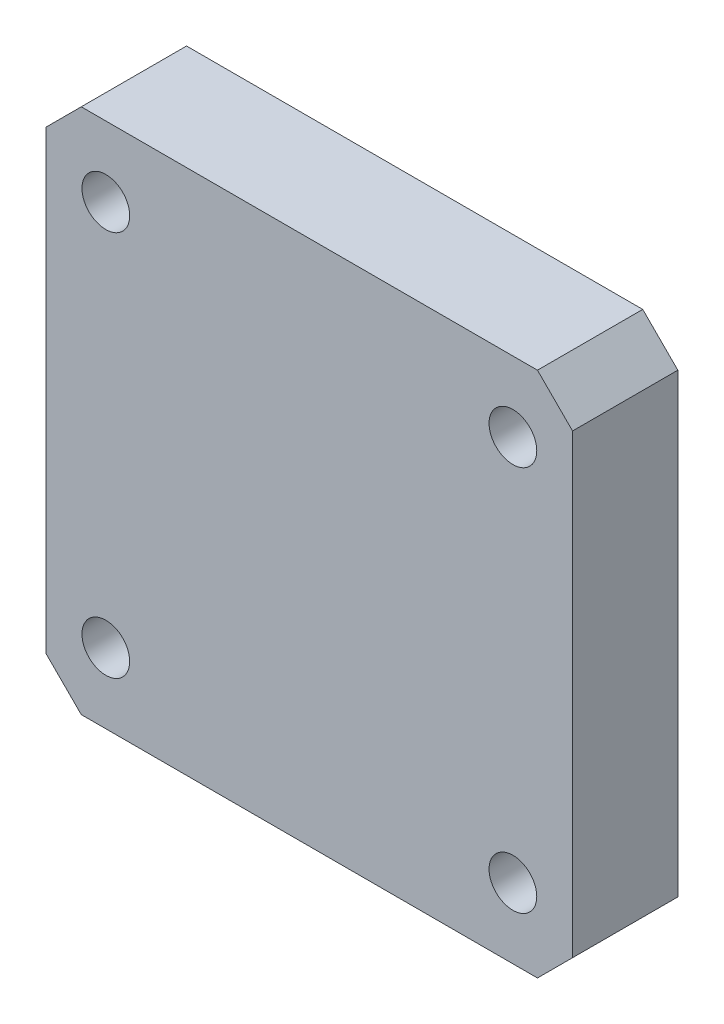
SolidWorks part; units mm, degrees
material "1023 碳钢板 (SS)"
ref_plane "Front Plane" through (0, 0, 0) normal (0, 0, 1) x (1, 0, 0)
ref_plane "Top Plane" through (0, 0, 0) normal (0, 1, 0) x (1, 0, 0)
ref_plane "Right Plane" through (0, 0, 0) normal (1, 0, 0) x (0, 0, -1)
sketch "Sketch1" plane through (0, 0, 0) normal (0, 0, 1) x (1, 0, 0)
  line L0 (-37.5, 32.5) -> (-32.5, 37.5)
  line L1 (-32.5, 37.5) -> (32.5, 37.5)
  line L2 (-37.5, 32.5) -> (-37.5, -32.5)
  line L3 (-32.5, -37.5) -> (32.5, -37.5)
  line L4 (37.5, 32.5) -> (37.5, -32.5)
  line L5 (-37.5, 37.5) -> (37.5, -37.5) construction
  line L6 (-37.5, -37.5) -> (37.5, 37.5) construction
  line L7 (32.5, 37.5) -> (37.5, 32.5)
  line L8 (32.5, -37.5) -> (37.5, -32.5)
  line L9 (-37.5, -32.5) -> (-32.5, -37.5)
  point P0 (0, 0)
  dimension "D1" = 75
  dimension "D2" = 75
extrude "Boss-Extrude1" add sketch "Sketch1" along normal blind 15
sketch "Sketch2" plane through (0, 0, 15) normal (0, 0, 1) x (1, 0, 0)
  line L1 (-29, 27.5) -> (29, 27.5) construction
  line L2 (-29, 27.5) -> (-29, -27.5) construction
  line L3 (-29, -27.5) -> (29, -27.5) construction
  line L4 (29, 27.5) -> (29, -27.5) construction
  line L5 (-29, 27.5) -> (29, -27.5) construction
  line L6 (-29, -27.5) -> (29, 27.5) construction
  point P0 (0, 0)
  dimension "D1" = 58
  dimension "D2" = 55
hole_wizard "M8 Tapped Hole1" positions "Sketch3" profile "Sketch4" tap size "M8" standard "GB"
sketch "Sketch3" plane through (0, 0, 15) normal (0, 0, 1) x (1, 0, 0)
  point P0 (-29, 27.5)
  point P3 (29, 27.5)
  point P6 (29, -27.5)
  point P9 (-29, -27.5)
sketch "Sketch4" plane through (-29, 27.5, 15) normal (1, 0, 0) x (0, -1, 0)
  line L0 (0, 0) -> (0, 21.7929)
  line L1 (0, 21.7929) -> (3.4, 19.75)
  line L2 (3.4, 19.75) -> (3.4, 0)
  line L5 (3.4, 0) -> (0, 0)
  line L10 (0, 21.7929) -> (-3.4, 19.75) construction
  line L11 (0, -6.35) -> (0, 107.95) construction
  dimension "螺纹孔钻头直径" = 6.8
  dimension "螺纹孔钻头深度" = 19.75
  dimension "导头角度" = 118
cosmetic thread "CosmeticThread Hole thread1"
cosmetic thread "CosmeticThread Hole thread2"
cosmetic thread "CosmeticThread Hole thread3"
cosmetic thread "CosmeticThread Hole thread4"
